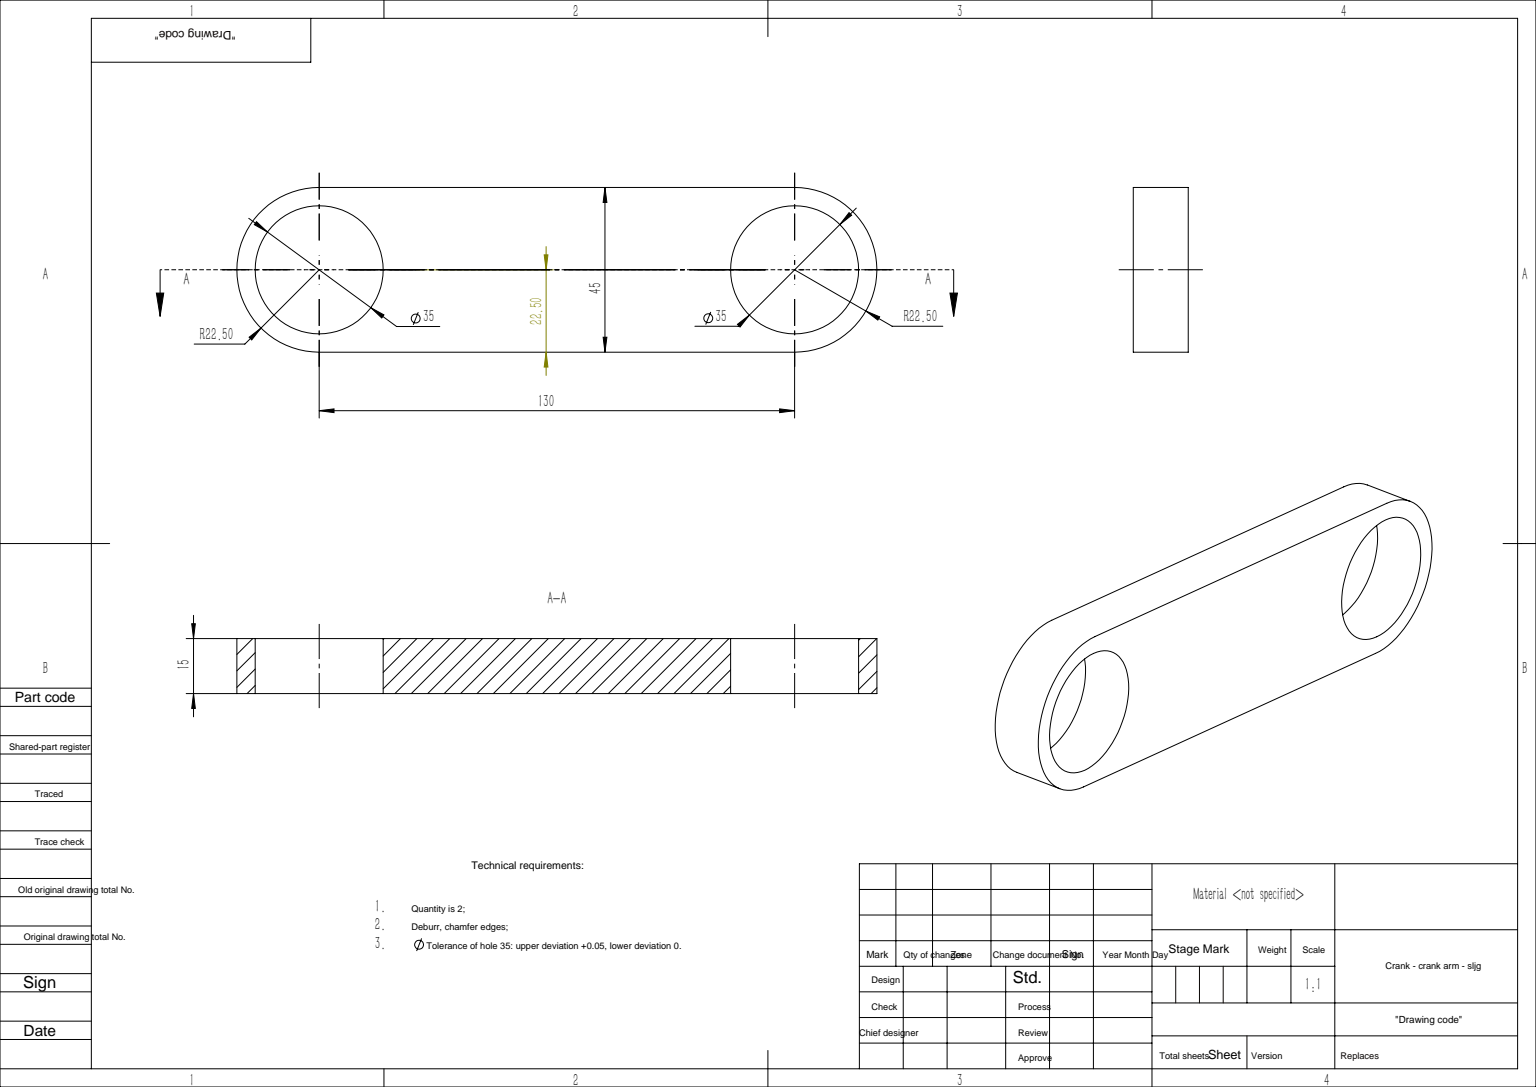
from build123d import *

# Parameters (mm, degrees)
EXTRUDE_1_DEPTH     = 15
SKETCH_2_R          = 17.5
CUT_EXTRUDE_1_DEPTH = 155.878985017
SKETCH_3_R          = 17.5
CUT_EXTRUDE_2_DEPTH = 155.878985017


with BuildPart() as part:
    # 草图1 → 凸台-拉伸1 (new body)
    with BuildSketch(Plane(origin=(0, 0, 0), x_dir=(0, 0, -1), z_dir=(1, 0, 0))):
        with BuildLine():
            Line((22.5, 0), (22.5, -130))
            ThreePointArc((22.5, -130), (0, -152.5), (-22.5, -130))
            Line((-22.5, -130), (-22.5, 0))
            ThreePointArc((-22.5, 0), (0, 22.5), (22.5, 0))
        make_face()
    extrude(amount=EXTRUDE_1_DEPTH)

    # 草图2 → 切除-拉伸1 (cut, through all)
    with BuildSketch(Plane(origin=(15, 0, 0), x_dir=(0, 0, -1), z_dir=(1, 0, 0))):
        Circle(SKETCH_2_R)
    extrude(amount=-CUT_EXTRUDE_1_DEPTH, mode=Mode.SUBTRACT)

    # 草图3 → 切除-拉伸2 (cut, through all)
    with BuildSketch(Plane.ZY):
        with Locations((0, -130)):
            Circle(SKETCH_3_R)
    extrude(amount=-CUT_EXTRUDE_2_DEPTH, mode=Mode.SUBTRACT)


solid = part.part
